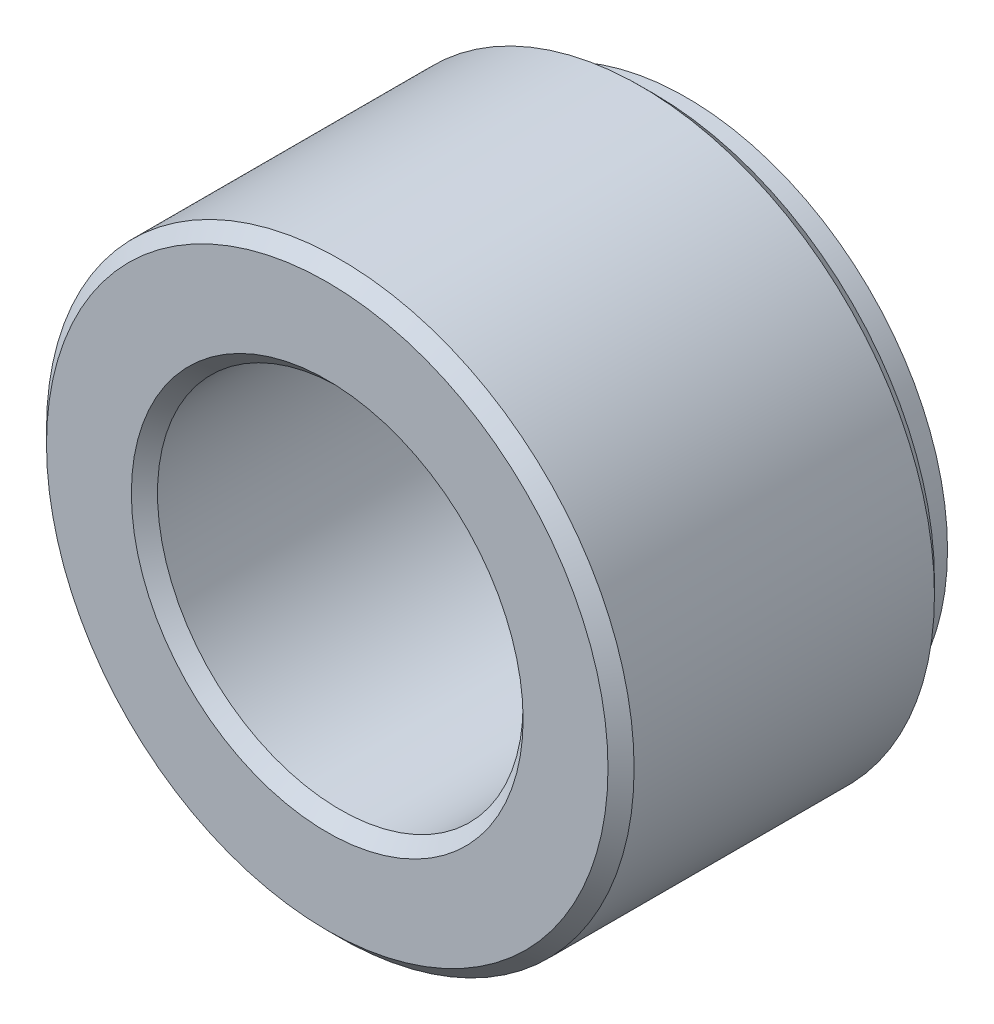
SolidWorks part; units mm, degrees
ref_plane "Front Plane" through (0, 0, 0) normal (0, 0, 1) x (1, 0, 0)
ref_plane "Top Plane" through (0, 0, 0) normal (0, 1, 0) x (1, 0, 0)
ref_plane "Right Plane" through (0, 0, 0) normal (1, 0, 0) x (0, 0, -1)
sketch "Sketch8" plane through (0, 0, 0) normal (0, 0, 1) x (1, 0, 0)
  circle A0 centre (-69.421, 0) radius 22.5
extrude "Boss-Extrude2" add sketch "Sketch8" along normal blind 25
sketch "Sketch9" plane through (0, 0, 25) normal (0, 0, 1) x (1, 0, 0)
  circle A0 centre (-69.421, 0) radius 13.1929
hole_wizard "M30x2.0 Tapped Hole1" positions "3DSketch6" profile "Sketch10" tap size "M30x2.0" standard "Ansi Metric"
sketch3d "3DSketch6"
  point P0 (-69.421, 0, 25)
sketch "Sketch10" plane through (-69.421, 0, 25) normal (1, 0, 0) x (0, -1, 0)
  line L0 (0, 0) -> (0, 78.412)
  line L1 (0, 78.412) -> (14, 70)
  line L2 (14, 70) -> (14, 0)
  line L5 (14, 0) -> (0, 0)
  line L10 (0, 78.412) -> (-14, 70) construction
  line L11 (0, -6.35) -> (0, 107.95) construction
  dimension "螺纹孔钻头直径" = 28
  dimension "螺纹孔钻头深度" = 70
  dimension "导头角度" = 118
cosmetic thread "Cosmetic thread 1" parameters "D1"=25, "D2"=30
sketch "Sketch11" plane through (0, 0, 0) normal (0, 0, -1) x (-1, 0, 0)
  circle A0 centre (69.421, 0) radius 20
  circle A1 centre (69.421, 0) radius 14
extrude "Boss-Extrude3" add sketch "Sketch11" along normal blind 2.5
chamfer "Chamfer1" distance 1 angle 45 3 edges at (-55.421, 0, 25) (-46.921, 0, 0) (-46.921, 0, 25)
